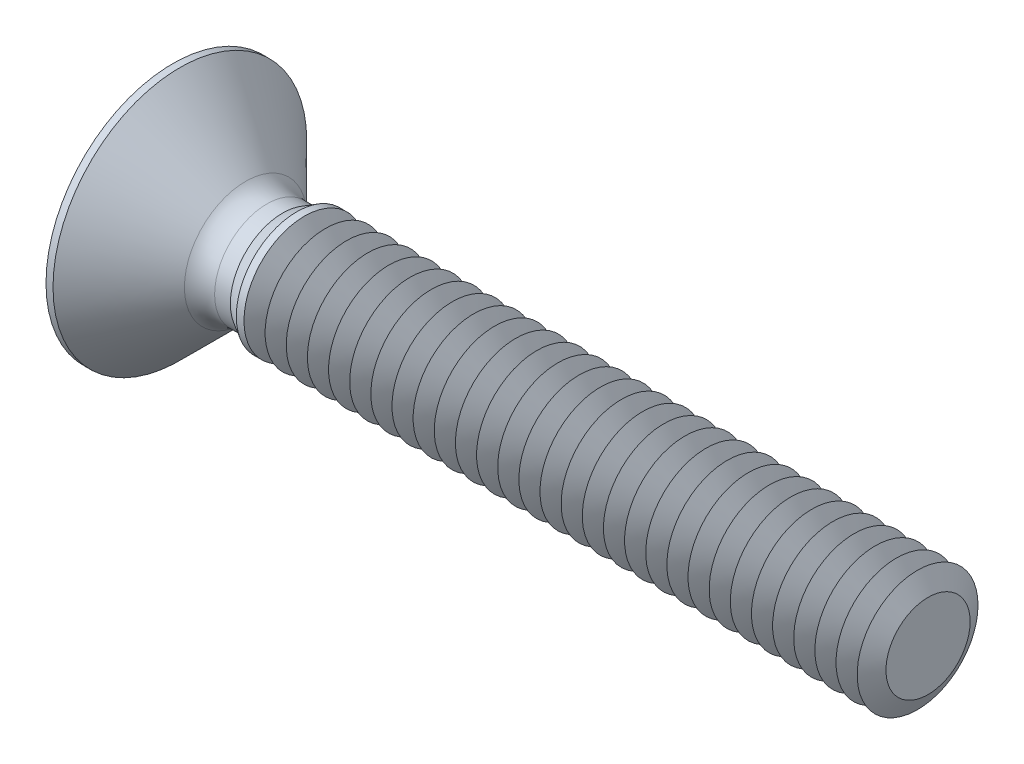
from build123d import *

# Parameters (mm, degrees)
PATTERN_LINEAR_1_COUNT   = 30
PATTERN_LINEAR_1_PITCH   = 0.7
PATTERN_CIRCULAR_1_COUNT = 2
PATTERN_CIRCULAR_1_ANGLE = 90


with BuildPart() as part:
    # 草图1 → Revolve 689 (revolve)
    with BuildSketch(Plane.XY, mode=Mode.PRIVATE) as revolve_689_sk:
        with BuildLine():
            Line((0, 0), (0, 4.2))
            Line((0, 4.2), (0.232, 4.2))
            Line((0.232, 4.2), (2.407106781, 2.024893219))
            ThreePointArc((2.407106781, 2.024893219), (2.73153013, 1.808120467), (3.114213562, 1.732))
            Line((3.114213562, 1.732), (3.635810384, 1.732))
            Line((3.635810384, 1.732), (4.1, 2))
            Line((4.1, 2), (25, 2))
            Line((25, 2), (25, 0))
            Line((25, 0), (0, 0))
        make_face()
    revolve(revolve_689_sk.sketch.rotate(Axis((0, 0, 0), (1, 0, 0)), 90), axis=Axis((0, 0, 0), (1, 0, 0)))

    # 草图2 → 切除-旋转1 (revolve, cut)
    with BuildSketch(Plane.XY, mode=Mode.PRIVATE) as cut_revolve_1_sk:
        Polygon((24.653791204, 2), (25.353791204, 2), (25, 1.3938), align=None)
    cut_revolve_1 = revolve(cut_revolve_1_sk.sketch.rotate(Axis((0, 0, 0), (-1, 0, 0)), 270), axis=Axis((0, 0, 0), (-1, 0, 0)), mode=Mode.SUBTRACT)

    # 阵列(线性)1: 切除-旋转1 ×30
    with Locations(*[(-i * PATTERN_LINEAR_1_PITCH, 0, 0) for i in range(1, PATTERN_LINEAR_1_COUNT)]):
        add(cut_revolve_1, mode=Mode.SUBTRACT)

    # 草图3 → 切除-放样1 section 0
    with BuildSketch(Plane.ZY, mode=Mode.PRIVATE) as loft_1_s0:
        with BuildLine():
            Line((-2.3, 0.35), (2.3, 0.35))
            Line((2.3, 0.35), (2.3, -0.35))
            Line((2.3, -0.35), (-2.3, -0.35))
            Line((-2.3, -0.35), (-2.3, 0.35))
        make_face()
    loft_1 = loft([loft_1_s0.sketch, Vertex(2.6, 0, 0)], mode=Mode.SUBTRACT)

    # 阵列(圆周)1: 切除-放样1 ×2 about axis
    pattern_circular_1_axis = Axis((0, 0, 0), (1, 0, 0))
    for i in range(1, PATTERN_CIRCULAR_1_COUNT):
        add(loft_1.rotate(pattern_circular_1_axis, i * PATTERN_CIRCULAR_1_ANGLE / (PATTERN_CIRCULAR_1_COUNT - 1)), mode=Mode.SUBTRACT)


solid = part.part
